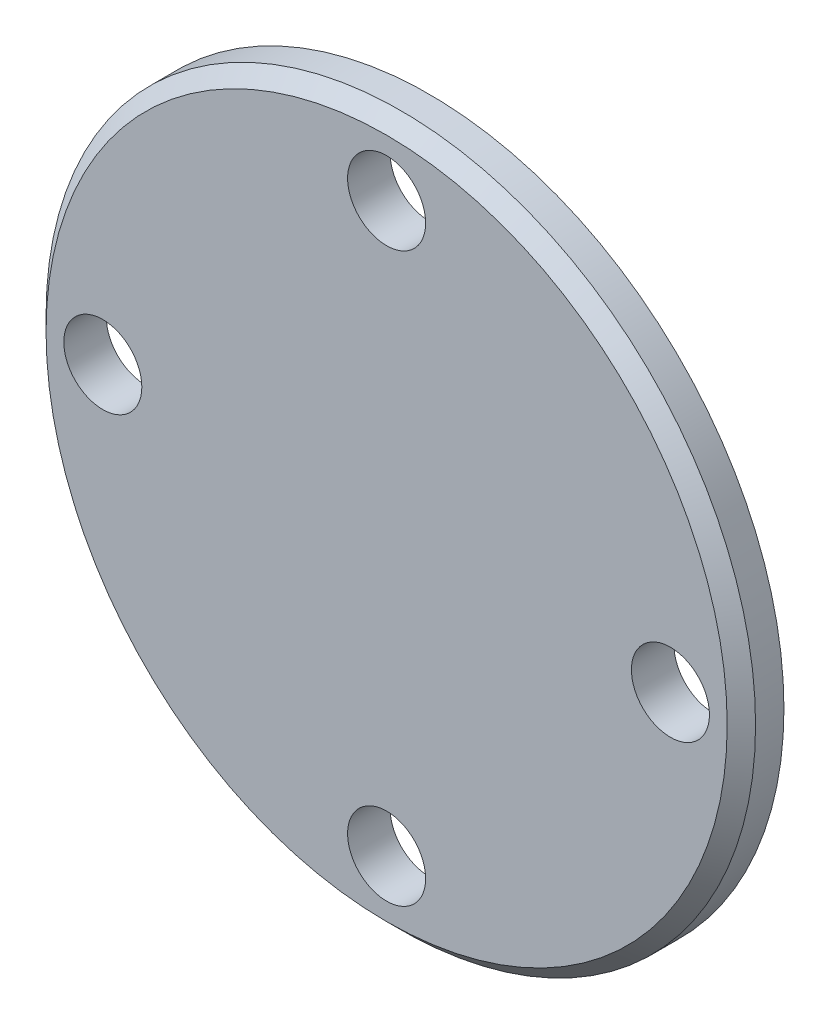
from build123d import *

# Parameters (mm, degrees)
SKETCH1_R           = 25
BOSS_EXTRUDE1_DEPTH = 3
CHAMFER1_SIZE       = 1
SKETCH2_R           = 2.75
CUT_EXTRUDE1_DEPTH  = 3


with BuildPart() as part:
    # Sketch1 → Boss-Extrude1 (new body)
    with BuildSketch(Plane.XY):
        Circle(SKETCH1_R)
    extrude(amount=BOSS_EXTRUDE1_DEPTH)

    # Chamfer1
    chamfer1_edges = [part.edges().sort_by_distance(p)[0] for p in [
        (-25, 0, 3),
    ]]
    chamfer(chamfer1_edges, length=CHAMFER1_SIZE)

    # Sketch2 → Cut-Extrude1 (cut)
    with BuildSketch(Plane.XY.offset(3)):
        with Locations((20, 0)):
            Circle(SKETCH2_R)
        with Locations((0, -20)):
            Circle(SKETCH2_R)
        with Locations((-20, 0)):
            Circle(SKETCH2_R)
        with Locations((0, 20)):
            Circle(SKETCH2_R)
    extrude(amount=-CUT_EXTRUDE1_DEPTH, mode=Mode.SUBTRACT)


solid = part.part
